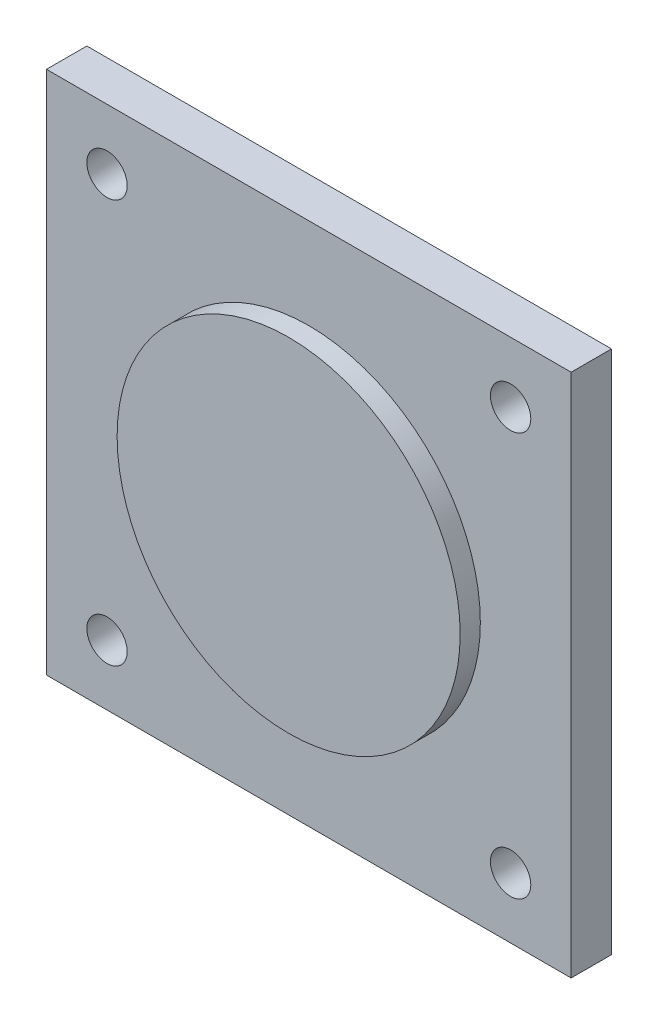
SolidWorks part; units mm, degrees
ref_plane "Front Plane" through (0, 0, 0) normal (0, 0, 1) x (1, 0, 0)
ref_plane "Top Plane" through (0, 0, 0) normal (0, 1, 0) x (1, 0, 0)
ref_plane "Right Plane" through (0, 0, 0) normal (1, 0, 0) x (0, 0, -1)
sketch "Sketch1" plane through (0, 0, 0) normal (0, 0, 1) x (1, 0, 0)
  line L1 (-65, 65) -> (65, 65)
  line L2 (-65, 65) -> (-65, -65)
  line L3 (-65, -65) -> (65, -65)
  line L4 (65, 65) -> (65, -65)
  line L5 (-65, 65) -> (65, -65) construction
  line L6 (-65, -65) -> (65, 65) construction
  point P0 (0, 0)
  dimension "D1" = 130
  dimension "D2" = 130
extrude "Boss-Extrude1" add sketch "Sketch1" along normal blind 10
sketch "Sketch2" plane through (0, 0, 10) normal (0, 0, 1) x (1, 0, 0)
  circle A0 centre (0, 0) radius 42.5
  dimension "D1" = 85
extrude "Boss-Extrude2" add sketch "Sketch2" along normal blind 5
sketch "Sketch3" plane through (0, 0, 10) normal (0, 0, 1) x (1, 0, 0)
  line L8 (50, -50) -> (50, 50)
  line L9 (50, 50) -> (-50, 50)
  line L10 (-50, 50) -> (-50, -50)
  line L11 (-50, -50) -> (50, -50)
  line L12 (50, -50) -> (50, 50) construction
  line L13 (50, 50) -> (-50, 50) construction
  line L14 (-50, 50) -> (-50, -50) construction
  line L15 (-50, -50) -> (50, -50) construction
  circle A0 centre (50, 50) radius 5
  circle A1 centre (-50, 50) radius 5
  circle A2 centre (-50, -50) radius 5
  circle A3 centre (50, -50) radius 5
  dimension "D2" = 10
  dimension "D1" = 15
extrude "Cut-Extrude1" cut sketch "Sketch3" against normal blind 51
